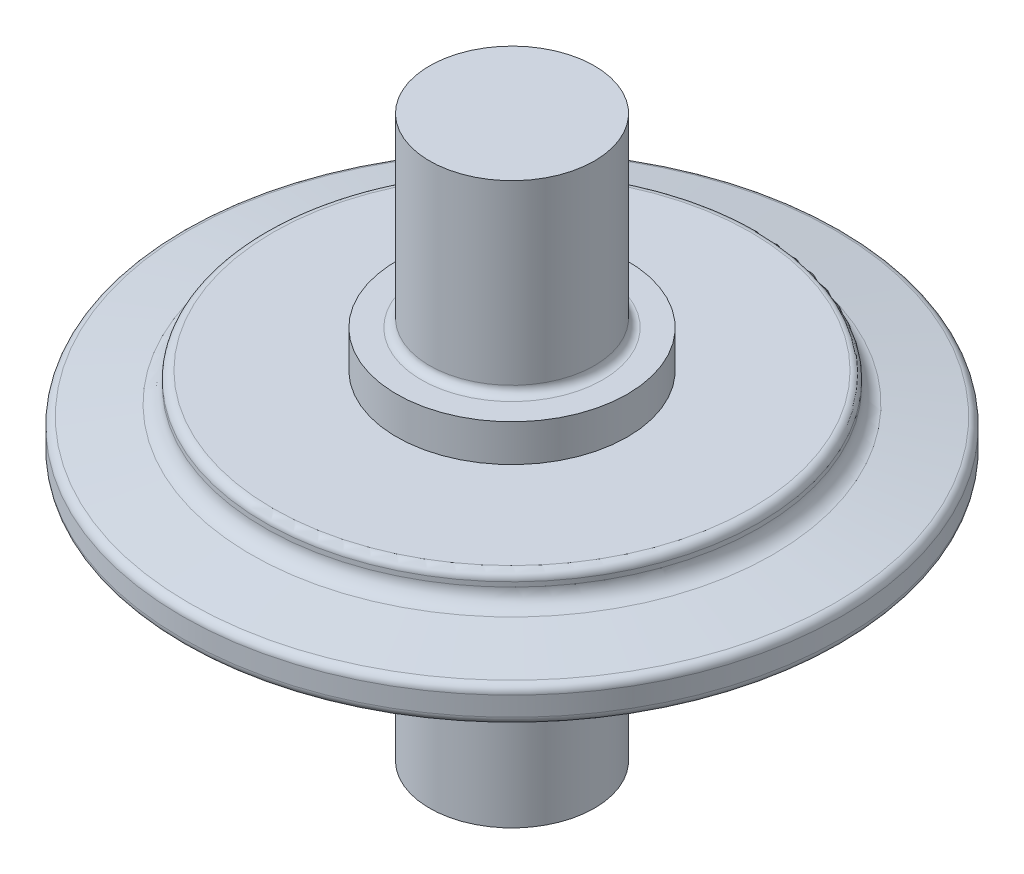
from build123d import *


with BuildPart() as part:
    # Sketch1 → Revolve1 (revolve)
    with BuildSketch(Plane.XY, mode=Mode.PRIVATE) as revolve1_sk:
        with BuildLine():
            Line((249.731774292, 31.667850424), (249.731774292, 29.346049686))
            ThreePointArc((249.731774292, 29.346049686), (249.965729849, 28.703262077), (250.558126114, 28.361241933))
            Line((250.558126114, 28.361241933), (258.079070647, 27.035096492))
            ThreePointArc((258.079070647, 27.035096492), (259.263863178, 26.351056205), (259.731774292, 25.065480986))
            Line((259.731774292, 25.065480986), (259.731774292, 24.506950055))
            ThreePointArc((259.731774292, 24.506950055), (260.024667511, 23.799843274), (260.731774292, 23.506950055))
            Line((260.731774292, 23.506950055), (275.731774292, 23.506950055))
            Line((275.731774292, 23.506950055), (275.731774292, 19.006950055))
            Line((275.731774292, 19.006950055), (278.731774292, 19.006950055))
            ThreePointArc((278.731774292, 19.006950055), (279.438881073, 18.714056836), (279.731774292, 18.006950055))
            Line((279.731774292, 18.006950055), (279.731774292, -3.493049945))
            Line((279.731774292, -3.493049945), (289.731774292, -3.493049945))
            Line((289.731774292, -3.493049945), (289.731774292, 64.506950055))
            Line((289.731774292, 64.506950055), (279.731774292, 64.506950055))
            Line((279.731774292, 64.506950055), (279.731774292, 43.006950055))
            ThreePointArc((279.731774292, 43.006950055), (279.438881073, 42.299843274), (278.731774292, 42.006950055))
            Line((278.731774292, 42.006950055), (275.731774292, 42.006950055))
            Line((275.731774292, 42.006950055), (275.731774292, 37.506950055))
            Line((275.731774292, 37.506950055), (260.731774292, 37.506950055))
            ThreePointArc((260.731774292, 37.506950055), (260.024667511, 37.214056836), (259.731774292, 36.506950055))
            Line((259.731774292, 36.506950055), (259.731774292, 35.948419125))
            ThreePointArc((259.731774292, 35.948419125), (259.263863178, 34.662843905), (258.079070647, 33.978803619))
            Line((258.079070647, 33.978803619), (250.558126114, 32.652658177))
            ThreePointArc((250.558126114, 32.652658177), (249.965729849, 32.310638034), (249.731774292, 31.667850424))
        make_face()
    revolve(revolve1_sk.sketch.rotate(Axis((289.731774292, -3.493049945, 0), (0, 1, 0)), 180), axis=Axis((289.731774292, -3.493049945, 0), (0, 1, 0)))


solid = part.part
